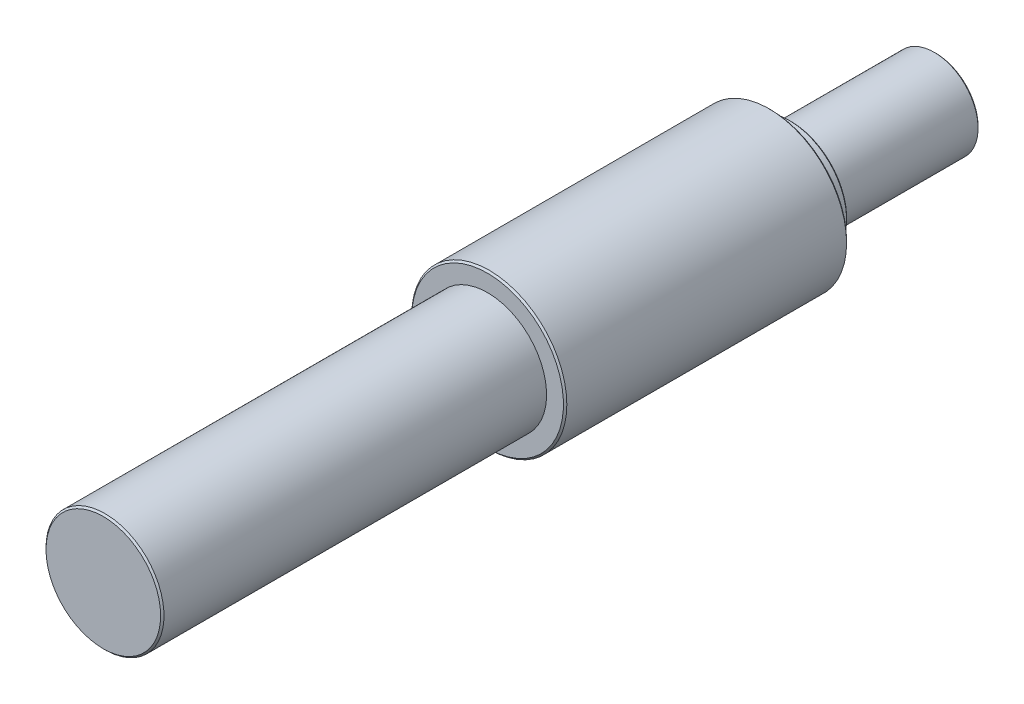
from build123d import *

# Parameters (mm, degrees)
SKETCH_1_R      = 17.5
EXTRUDE_1_DEPTH = 57
SKETCH_2_R      = 23
EXTRUDE_2_DEPTH = 84
SKETCH_3_R      = 17
EXTRUDE_3_DEPTH = 6
SKETCH_4_R      = 13
EXTRUDE_4_DEPTH = 43
CHAMFER_1_SIZE  = 0.5


with BuildPart() as part:
    # 草图1 → 凸台-拉伸1 (new, symmetric)
    with BuildSketch(Plane.XY):
        with Locations(Location((0, 0, 0), (0, 0, 180))):
            Circle(SKETCH_1_R)
    extrude(amount=EXTRUDE_1_DEPTH, both=True)

    # 草图2 → 凸台-拉伸2 (add)
    with BuildSketch(Plane(origin=(0, 0, -57), x_dir=(-1, 0, 0), z_dir=(0, 0, -1))):
        with Locations(Location((0, 0, 0), (0, 0, 180))):
            Circle(SKETCH_2_R)
    extrude(amount=EXTRUDE_2_DEPTH)

    # 草图3 → 凸台-拉伸3 (add)
    with BuildSketch(Plane(origin=(0, 0, -141), x_dir=(-1, 0, 0), z_dir=(0, 0, -1))):
        Circle(SKETCH_3_R)
    extrude(amount=EXTRUDE_3_DEPTH)

    # 草图4 → 凸台-拉伸4 (add)
    with BuildSketch(Plane(origin=(0, 0, -147), x_dir=(-1, 0, 0), z_dir=(0, 0, -1))):
        Circle(SKETCH_4_R)
    extrude(amount=EXTRUDE_4_DEPTH)

    # 倒角1
    chamfer_1_edges = [part.edges().sort_by_distance(p)[0] for p in [
        (17, 0, -147),
        (13, 0, -190),
        (17.5, 0, 57),
        (-23, 0, -57),
        (-23, 0, -141),
    ]]
    chamfer(chamfer_1_edges, length=CHAMFER_1_SIZE)


solid = part.part
